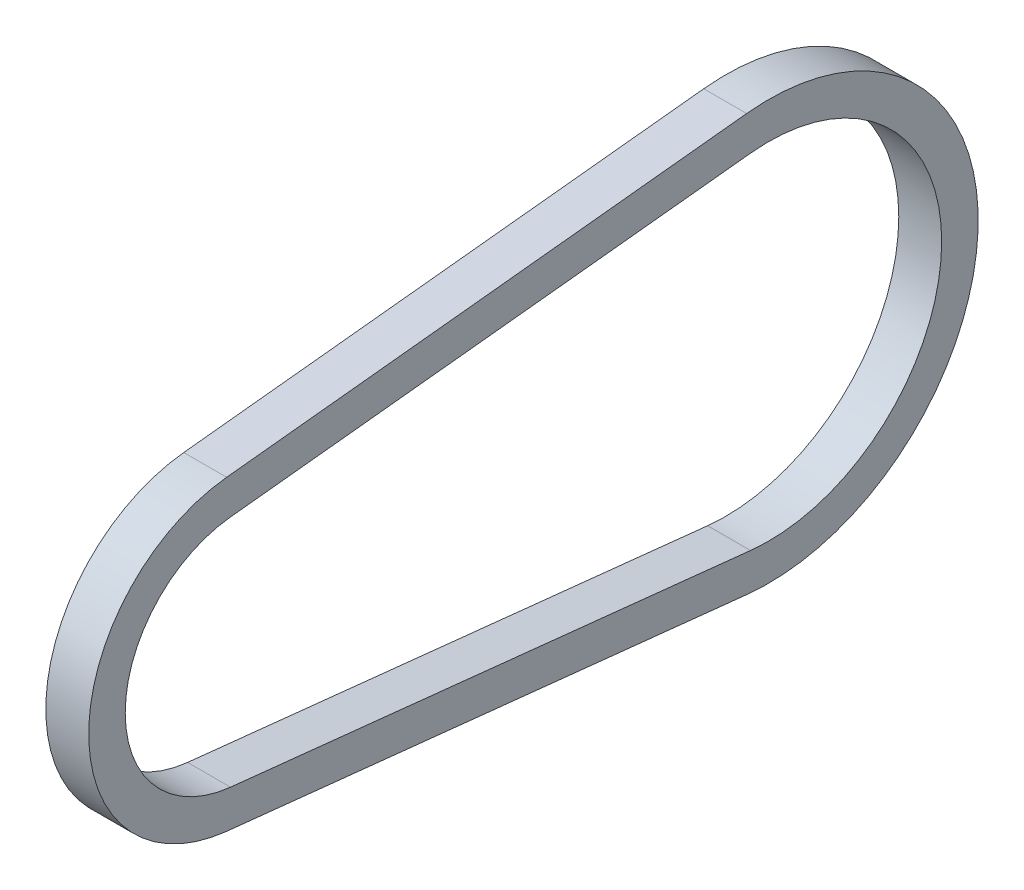
SolidWorks part; units mm, degrees
ref_plane "前视基准面" through (0, 0, 0) normal (0, 0, 1) x (1, 0, 0)
ref_plane "上视基准面" through (0, 0, 0) normal (0, 1, 0) x (1, 0, 0)
ref_plane "右视基准面" through (0, 0, 0) normal (1, 0, 0) x (0, 0, -1)
sketch "草图1" plane through (0, 0, 0) normal (1, 0, 0) x (0, 0, -1)
  line L0 (-87.8495, 35.3861) -> (139.9981, 59.5014)
  line L1 (-87.8495, -67.1412) -> (139.9981, -91.2565)
  arc A0 (-87.8495, 35.3861) -> (-87.8495, -67.1412) centre (-82.4238, -15.8775) ccw
  arc A1 (139.9981, -91.2565) -> (139.9981, 59.5014) centre (147.9762, -15.8775) ccw
  dimension "D1" = 151.6
  dimension "D2" = 103.1
  dimension "D3" = 230.4
extrude "拉伸-薄壁1" add sketch "草图1" along normal blind 18.8 thin thin type one direction wall 16
